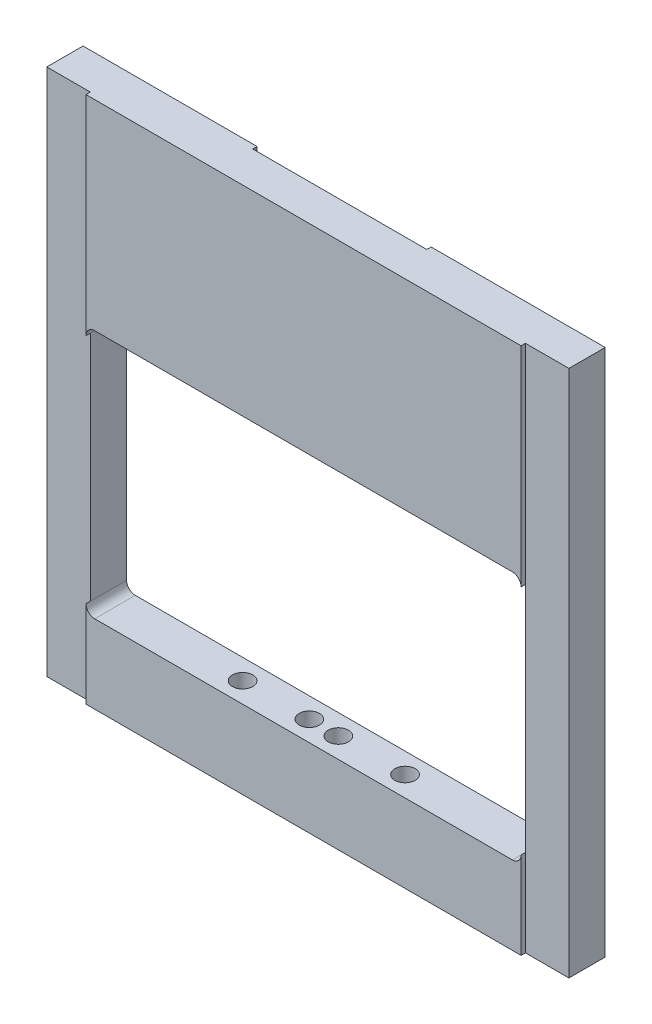
from build123d import *

# Parameters (mm, degrees)
SKETCH_1_W          = 180
SKETCH_1_H          = 182
EXTRUDE_1_DEPTH     = 7
SKETCH_2_W          = 60
SKETCH_2_H          = 64
SKETCH_2_H_2        = 22
CUT_EXTRUDE_1_DEPTH = 1.5
CUT_EXTRUDE_2_DEPTH = 1.5
CUT_EXTRUDE_3_REACH = 130.752
SKETCH_4_W          = 150
SKETCH_4_H          = 86
FILLET_1_R          = 3
CUT_EXTRUDE_4_REACH = 205.158
SKETCH_6_R          = 3.5
SKETCH_7_W          = 15
SKETCH_7_H          = 182
CUT_EXTRUDE_5_DEPTH = 1.5


with BuildPart() as part:
    # 草图1 → 凸台-拉伸1 (new, symmetric)
    with BuildSketch(Plane.XY):
        Rectangle(SKETCH_1_W, SKETCH_1_H)
    extrude(amount=EXTRUDE_1_DEPTH, both=True)

    # 草图2 → 切除-拉伸1 (cut)
    with BuildSketch(Plane(origin=(0, 0, -7), x_dir=(-1, 0, 0), z_dir=(0, 0, -1))):
        with Locations((0, 59)):
            Rectangle(SKETCH_2_W, SKETCH_2_H)
        with Locations((0, -80)):
            Rectangle(SKETCH_2_W, SKETCH_2_H_2)
    extrude(amount=-CUT_EXTRUDE_1_DEPTH, mode=Mode.SUBTRACT)

    # 草图3 → 切除-拉伸2 (cut)
    with BuildSketch(Plane(origin=(0, 0, -7), x_dir=(-1, 0, 0), z_dir=(0, 0, -1))):
        with BuildLine():
            Line((30, 27), (32, 27))
            ThreePointArc((32, 27), (37, 32), (32, 37))
            Line((32, 37), (30, 37))
            Line((30, 37), (30, 27))
        make_face()
        with BuildLine():
            Line((-30, 37), (-30, 27))
            Line((-30, 27), (-32, 27))
            ThreePointArc((-32, 27), (-37, 32), (-32, 37))
            Line((-32, 37), (-30, 37))
        make_face()
        with BuildLine():
            Line((30, -69), (32, -69))
            ThreePointArc((32, -69), (37, -74), (32, -79))
            Line((32, -79), (30, -79))
            Line((30, -79), (30, -69))
        make_face()
        with BuildLine():
            Line((-30, -79), (-30, -69))
            Line((-30, -69), (-32, -69))
            ThreePointArc((-32, -69), (-37, -74), (-32, -79))
            Line((-32, -79), (-30, -79))
        make_face()
    extrude(amount=-CUT_EXTRUDE_2_DEPTH, mode=Mode.SUBTRACT)

    # 草图4 → 切除-拉伸3 (cut, up to next)
    with BuildSketch(Plane(origin=(0, 0, -7), x_dir=(-1, 0, 0), z_dir=(0, 0, -1)), mode=Mode.PRIVATE) as cut_extrude_3_sk1:
        with Locations((0, -21)):
            Rectangle(SKETCH_4_W, SKETCH_4_H)
    cut_extrude_3_tool1 = extrude(cut_extrude_3_sk1.sketch, amount=-CUT_EXTRUDE_3_REACH, mode=Mode.PRIVATE) & part.part
    add(cut_extrude_3_tool1.solids().sort_by_distance((0, -21, -7))[0], mode=Mode.SUBTRACT)

    # 圆角1
    fillet_1_edges = [part.edges().sort_by_distance(p)[0] for p in [
        (-75, 22, 0),
        (-75, -64, 0),
        (75, -64, 0),
        (75, 22, 0),
    ]]
    fillet(fillet_1_edges, radius=FILLET_1_R)

    # 草图6 → 切除-拉伸4 (cut, up to next)
    with BuildSketch(Plane.XZ.offset(91), mode=Mode.PRIVATE) as cut_extrude_4_sk1:
        with Locations(Location((-28, 0, 0), (0, 0, 270))):
            Circle(SKETCH_6_R)
    cut_extrude_4_tool1 = extrude(cut_extrude_4_sk1.sketch, amount=-CUT_EXTRUDE_4_REACH, mode=Mode.PRIVATE) & part.part
    # 草图6 → 切除-拉伸4 (cut, up to next)
    with BuildSketch(Plane.XZ.offset(91), mode=Mode.PRIVATE) as cut_extrude_4_sk2:
        with Locations(Location((28, 0, 0), (0, 0, 270))):
            Circle(SKETCH_6_R)
    cut_extrude_4_tool2 = extrude(cut_extrude_4_sk2.sketch, amount=-CUT_EXTRUDE_4_REACH, mode=Mode.PRIVATE) & part.part
    # 草图6 → 切除-拉伸4 (cut, up to next)
    with BuildSketch(Plane.XZ.offset(91), mode=Mode.PRIVATE) as cut_extrude_4_sk3:
        with Locations(Location((-5, 0, 0), (0, 0, 270))):
            Circle(SKETCH_6_R)
    cut_extrude_4_tool3 = extrude(cut_extrude_4_sk3.sketch, amount=-CUT_EXTRUDE_4_REACH, mode=Mode.PRIVATE) & part.part
    # 草图6 → 切除-拉伸4 (cut, up to next)
    with BuildSketch(Plane.XZ.offset(91), mode=Mode.PRIVATE) as cut_extrude_4_sk4:
        with Locations(Location((5, 0, 0), (0, 0, 270))):
            Circle(SKETCH_6_R)
    cut_extrude_4_tool4 = extrude(cut_extrude_4_sk4.sketch, amount=-CUT_EXTRUDE_4_REACH, mode=Mode.PRIVATE) & part.part
    add(cut_extrude_4_tool1.solids().sort_by_distance((-28, -91, 0))[0], mode=Mode.SUBTRACT)
    add(cut_extrude_4_tool2.solids().sort_by_distance((28, -91, 0))[0], mode=Mode.SUBTRACT)
    add(cut_extrude_4_tool3.solids().sort_by_distance((-5, -91, 0))[0], mode=Mode.SUBTRACT)
    add(cut_extrude_4_tool4.solids().sort_by_distance((5, -91, 0))[0], mode=Mode.SUBTRACT)

    # 草图7 → 切除-拉伸5 (cut)
    with BuildSketch(Plane.XY.offset(7)):
        with Locations((-82.5, 0)):
            Rectangle(SKETCH_7_W, SKETCH_7_H)
        with Locations((82.5, 0)):
            Rectangle(SKETCH_7_W, SKETCH_7_H)
    extrude(amount=-CUT_EXTRUDE_5_DEPTH, mode=Mode.SUBTRACT)


solid = part.part
